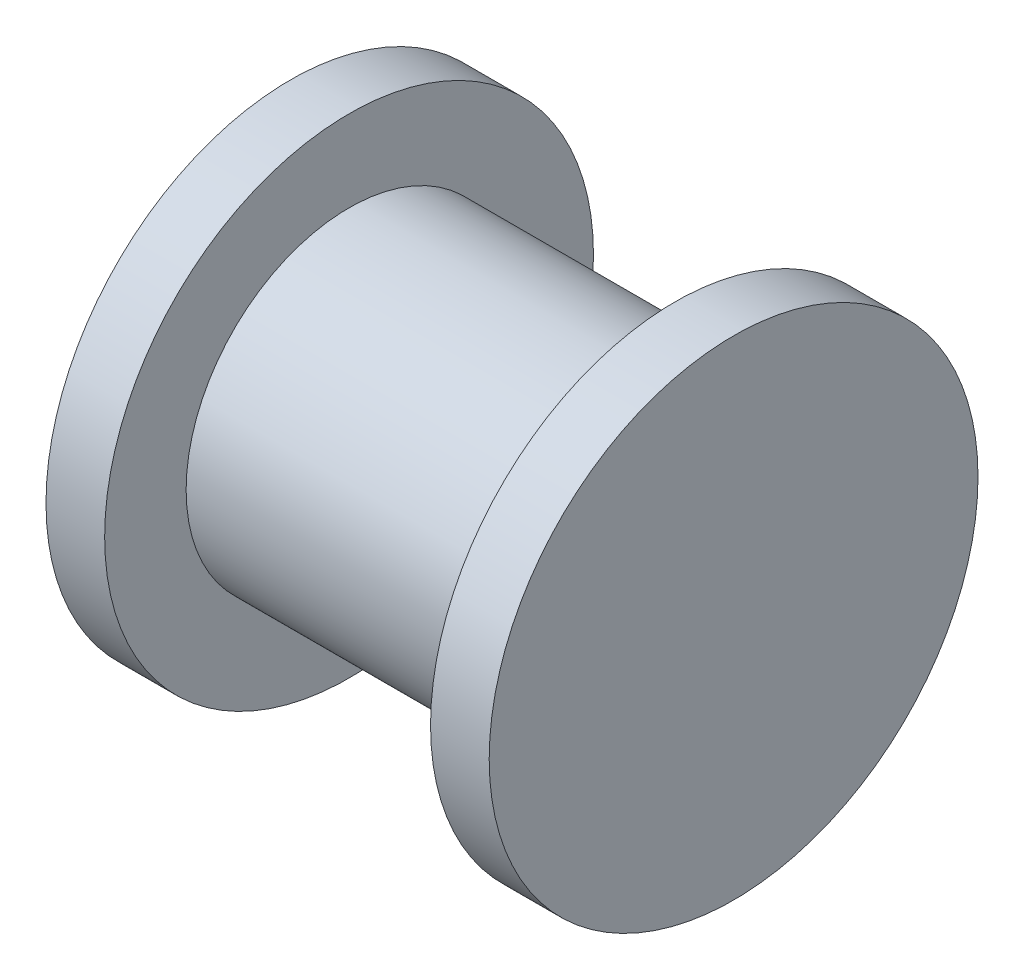
from build123d import *

# Parameters (mm, degrees)
SKETCH_1_4_R        = 75
BOSS_EXTRUDE1_DEPTH = 18
SKETCH_1_3_R        = 50
BOSS_EXTRUDE2_DEPTH = 100
BOSS_EXTRUDE3_START = -118
SKETCH_1_4_2_R      = 75
BOSS_EXTRUDE3_DEPTH = 18


with BuildPart() as part:
    # Sketch 1_4 → Boss-Extrude1 (new body)
    with BuildSketch(Plane(origin=(0, 0, 0), x_dir=(0, 0, -1), z_dir=(1, 0, 0))):
        Circle(SKETCH_1_4_R)
    extrude(amount=BOSS_EXTRUDE1_DEPTH)

    # 草图1<3> → Boss-Extrude2 (add)
    with BuildSketch(Plane(origin=(0, 0, 0), x_dir=(0, 0, -1), z_dir=(1, 0, 0))):
        Circle(SKETCH_1_3_R)
    extrude(amount=-BOSS_EXTRUDE2_DEPTH)

    # Sketch 1_4 2 → Boss-Extrude3 (add)
    with BuildSketch(Plane(origin=(0, 0, 0), x_dir=(0, 0, -1), z_dir=(1, 0, 0)).offset(BOSS_EXTRUDE3_START)):
        Circle(SKETCH_1_4_2_R)
    extrude(amount=BOSS_EXTRUDE3_DEPTH)


solid = part.part
